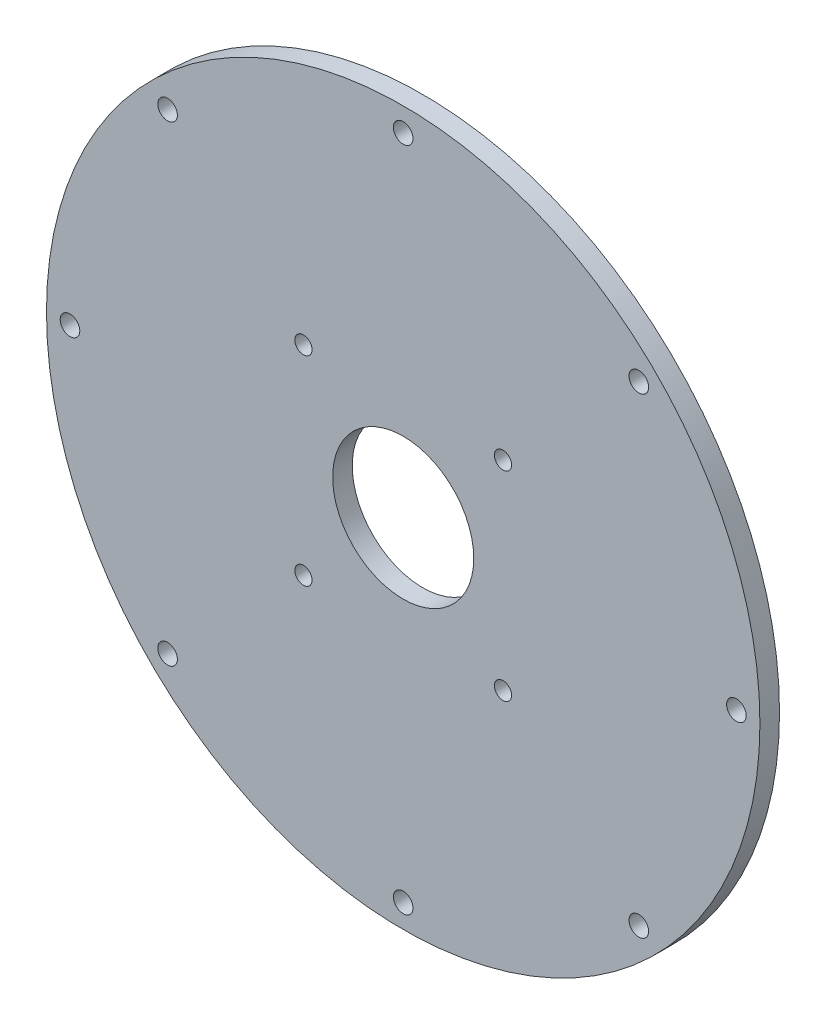
SolidWorks part; units mm, degrees
ref_plane "前视基准面" through (0, 0, 0) normal (0, 0, 1) x (1, 0, 0)
ref_plane "上视基准面" through (0, 0, 0) normal (0, 1, 0) x (1, 0, 0)
ref_plane "右视基准面" through (0, 0, 0) normal (1, 0, 0) x (0, 0, -1)
sketch "草图1" plane through (0, 0, 0) normal (0, 0, 1) x (1, 0, 0)
  circle A0 centre (0, 0) radius 18
  circle A1 centre (0, 0) radius 91
  dimension "D1" = 36
  dimension "D2" = 182
extrude "凸台-拉伸1" add sketch "草图1" along normal mid plane 5
sketch "草图2" plane through (0, 0, 2.5) normal (0, 0, 1) x (1, 0, 0)
  line L0 (0, 85) -> (0, 0) construction
  circle A0 centre (0, 85) radius 2.5
  dimension "D1" = 5
  dimension "D2" = 85
extrude "切除-拉伸1" cut sketch "草图2" against normal blind 5
pattern_circular "阵列(圆周)1" count 8 over 360 about axis through (0, 0, 0) along (0, 0, 1) of "切除-拉伸1"
sketch "草图3" plane through (0, 0, -2.5) normal (0, 0, -1) x (-1, 0, 0)
  line L0 (0, 0) -> (25.4558, 25.4558) construction
  line L1 (0, 0) -> (31.2476, 0) construction
  circle A0 centre (25.4558, 25.4558) radius 2.2
  dimension "D1" = 4.4
  dimension "D2" = 36
  dimension "D3" = 45
extrude "切除-拉伸2" cut sketch "草图3" against normal blind 10
pattern_circular "阵列(圆周)2" count 4 over 360 about axis through (0, 0, 0) along (0, 0, 1) of "切除-拉伸2"
